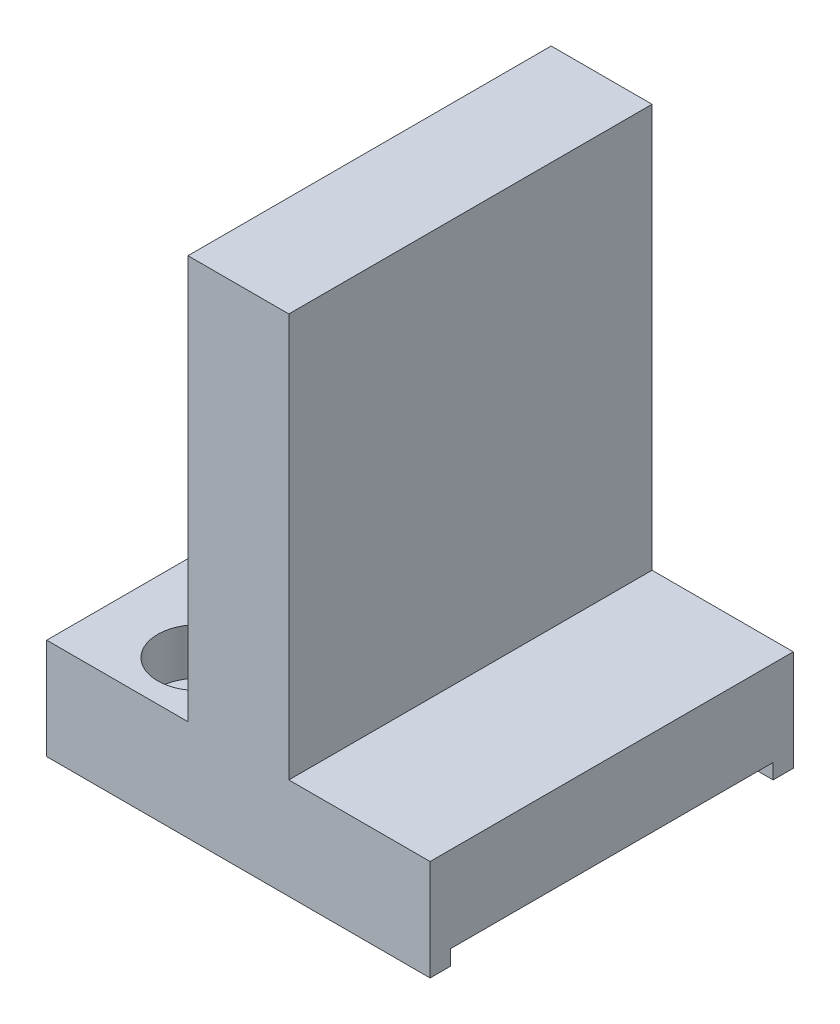
SolidWorks part; units mm, degrees
ref_plane "前视基准面" through (0, 0, 0) normal (0, 0, 1) x (1, 0, 0)
ref_plane "上视基准面" through (0, 0, 0) normal (0, 1, 0) x (1, 0, 0)
ref_plane "右视基准面" through (0, 0, 0) normal (1, 0, 0) x (0, 0, -1)
sketch "草图1" plane through (0, 0, 0) normal (0, 0, 1) x (1, 0, 0)
  line L0 (0, 0) -> (-19, 0)
  line L1 (-19, 0) -> (-19, 10)
  line L2 (-19, 10) -> (-5, 10)
  line L3 (-5, 10) -> (-5, 50)
  line L4 (-5, 50) -> (5, 50)
  line L5 (5, 50) -> (5, 10)
  line L6 (5, 10) -> (19, 10)
  line L7 (19, 10) -> (19, 0)
  line L8 (19, 0) -> (0, 0)
  dimension "D1" = 10
  dimension "D2" = 38
  dimension "D3" = 10
  dimension "D4" = 40
extrude "凸台-拉伸1" add sketch "草图1" along normal mid plane 36
sketch "草图2" plane through (0, 0, 0) normal (0, -1, 0) x (1, 0, 0)
  line L0 (19, 18) -> (19, -18) construction
  line L1 (-19, 16) -> (19, 16)
  line L2 (-19, 16) -> (-19, -16)
  line L3 (-19, -16) -> (19, -16)
  line L4 (19, 16) -> (19, -16)
  line L5 (-19, 16) -> (19, -16) construction
  line L6 (-19, -16) -> (19, 16) construction
  point P0 (0, 0)
  dimension "D1" = 32
extrude "切除-拉伸1" cut sketch "草图2" against normal blind 1.5
hole_wizard "打孔尺寸(%根据)内六角圆柱头螺钉的类型1" positions "3D草图1" profile "草图3" counterbore size "M4" standard "GB" end condition up to next
sketch3d "3D草图1"
  circle A0 centre (-10, 1.5, 12) radius 2 construction
  point P0 (-10, 10, 12)
  point P5 (-10, 3.5, 12)
sketch "草图3" plane through (-10, 10, 12) normal (1, 0, 0) x (0, 0, 1)
  line L0 (0, 0) -> (0, 8.5)
  line L1 (0, 8.5) -> (2.25, 8.5)
  line L3 (2.25, 8.5) -> (2.25, 4.6)
  line L4 (2.25, 4.6) -> (4, 4.6)
  line L5 (4, 4.6) -> (4, 0)
  line L7 (4, 0) -> (0, 0)
  line L11 (0, -6.35) -> (0, 107.95) construction
  dimension "通孔孔直径" = 4.5
  dimension "通孔孔深度" = 8.5
  dimension "柱形沉头孔直径" = 8
  dimension "柱形沉头孔深度" = 4.6
